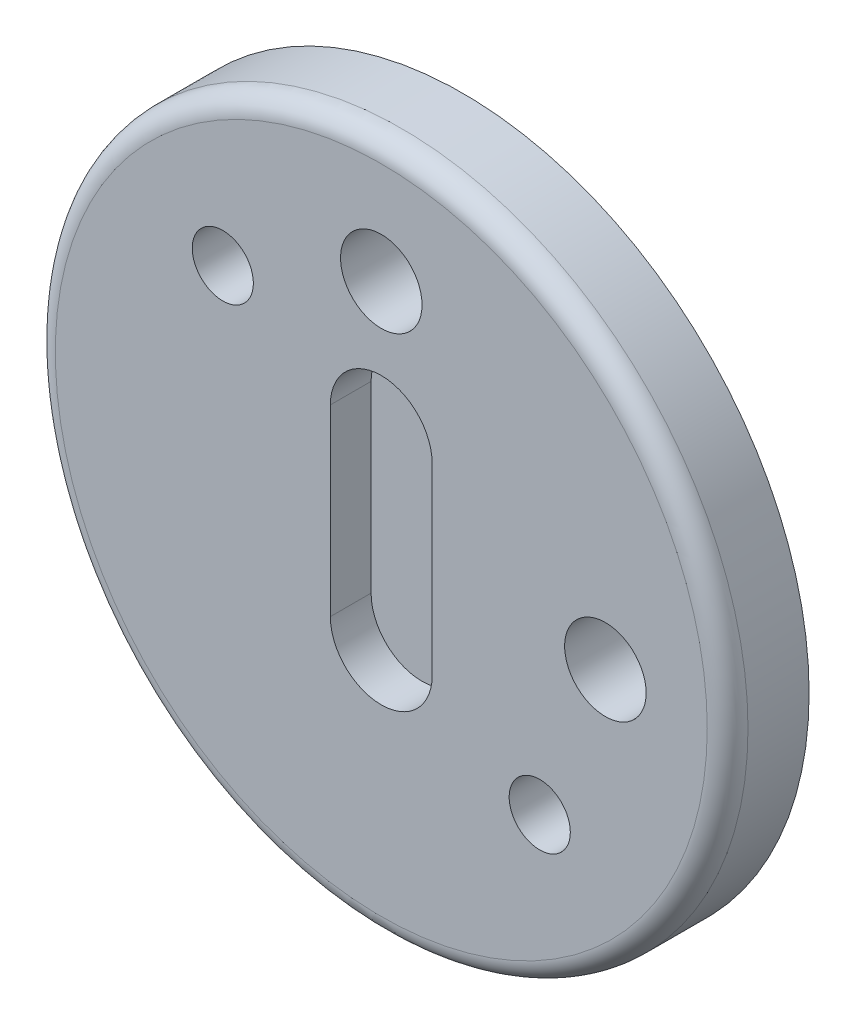
from build123d import *

# Parameters (mm, degrees)
SKETCH1_R           = 17
BOSS_EXTRUDE1_DEPTH = 4
CUT_EXTRUDE1_DEPTH  = 2
SKETCH3_R           = 2
SKETCH3_R_2         = 1.5
CUT_EXTRUDE2_DEPTH  = 4
FILLET1_R           = 1


with BuildPart() as part:
    # Sketch1 → Boss-Extrude1 (new body)
    with BuildSketch(Plane.XY):
        Circle(SKETCH1_R)
    extrude(amount=BOSS_EXTRUDE1_DEPTH)

    # Sketch2 → Cut-Extrude1 (cut)
    with BuildSketch(Plane.XY.offset(4)):
        with BuildLine():
            Line((2.5, 4.5), (2.5, -4.5))
            ThreePointArc((2.5, -4.5), (0, -7), (-2.5, -4.5))
            Line((-2.5, -4.5), (-2.5, 4.5))
            ThreePointArc((-2.5, 4.5), (0, 7), (2.5, 4.5))
        make_face()
    extrude(amount=-CUT_EXTRUDE1_DEPTH, mode=Mode.SUBTRACT)

    # Sketch3 → Cut-Extrude2 (cut)
    with BuildSketch(Plane.XY.offset(4)):
        with Locations((0, 11)):
            Circle(SKETCH3_R)
        with Locations((11, 0)):
            Circle(SKETCH3_R)
        with Locations((-7.778174593, 7.778174593)):
            Circle(SKETCH3_R_2)
        with Locations((7.778174593, -7.778174593)):
            Circle(SKETCH3_R_2)
    extrude(amount=-CUT_EXTRUDE2_DEPTH, mode=Mode.SUBTRACT)

    # Fillet1
    fillet1_edges = [part.edges().sort_by_distance(p)[0] for p in [
        (-17, 0, 4),
    ]]
    fillet(fillet1_edges, radius=FILLET1_R)


solid = part.part
